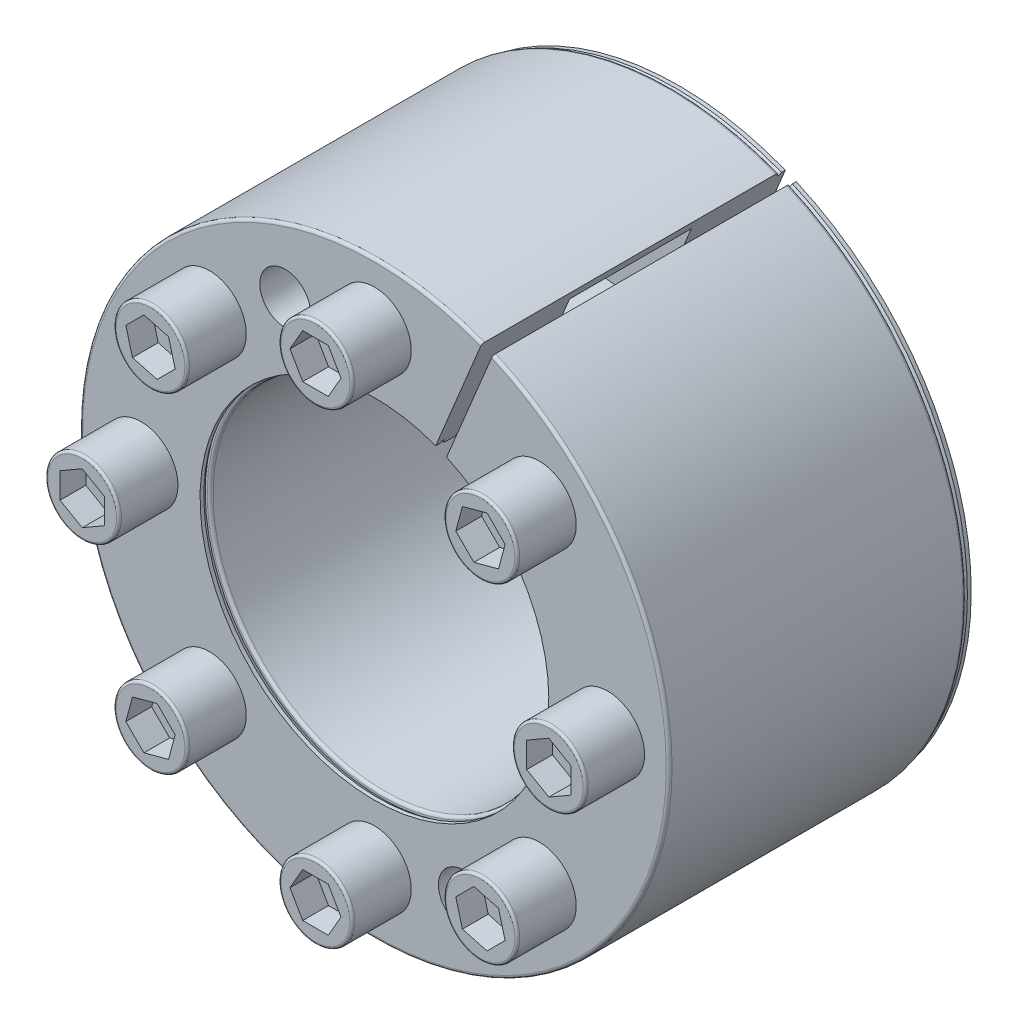
from build123d import *

# Parameters (mm, degrees)
SKETCH7_W                                 = 12.4
SKETCH7_H                                 = 10.625
FILLET2_R                                 = 0.3
SKETCH8_W                                 = 12.4
SKETCH8_H                                 = 3
SCREW_SKETCH1_R                           = 3.75
EXTRUDE_SCREW_SOCKET_HEAD_DEPTH           = 6
FILLET_SCREW_SOCKET_HEAD_R                = 0.25
CUT_SCREW_SOCKET_HEAD_DEPTH               = 2.625
SKETCH5_W                                 = 4.65
SKETCH5_H                                 = 3
CIRPATTERN1_COUNT                         = 8
FILLET_SCREW_SOCKET_HEAD_OF_CIRPATTERN1_R = 0.25
SKETCH6_R                                 = 2.57578125
CUT_EXTRUDE1_DEPTH                        = 9.3
CIRPATTERN2_COUNT                         = 2
CUT_EXTRUDE_THIN1_DEPTH                   = 53.545218679


with BuildPart() as part:
    # Sketch2 → Revolve1 (revolve)
    with BuildSketch(Plane(origin=(0, 0, 0), x_dir=(0, 0, -1), z_dir=(1, 0, 0)), mode=Mode.PRIVATE) as revolve1_sk:
        Polygon((0.775, 17.5), (31, 17.5), (31, 29.75), (30.6125, 29.75), (30.225, 29.5), (30.225, 30), (0, 30), (0, 18), (0, 17.75), (0.3875, 17.75), (0.775, 18), align=None)
    revolve(revolve1_sk.sketch.rotate(Axis((0, 0, 0), (0, 0, -1)), 90), axis=Axis((0, 0, 0), (0, 0, -1)))

    # Sketch7 → Cut-Revolve2 (revolve, cut)
    with BuildSketch(Plane(origin=(0, 0, 0), x_dir=(0, 0, -1), z_dir=(1, 0, 0)), mode=Mode.PRIVATE) as cut_revolve2_sk:
        with Locations((15.5, 23.75)):
            Rectangle(SKETCH7_W, SKETCH7_H)
    revolve(cut_revolve2_sk.sketch.rotate(Axis((0, 0, 0), (0, 0, -1)), 90), axis=Axis((0, 0, 0), (0, 0, -1)), mode=Mode.SUBTRACT)

    # Fillet2
    fillet2_edges = [part.edges().sort_by_distance(p)[0] for p in [
        (-30, 0, 0),
        (-30, 0, -30.225),
        (-17.5, 0, -31),
        (-17.5, 0, -0.775),
    ]]
    fillet(fillet2_edges, radius=FILLET2_R)

    # Sketch8 → Revolve2 (revolve)
    with BuildSketch(Plane(origin=(0, 0, 0), x_dir=(0, 0, -1), z_dir=(1, 0, 0)), mode=Mode.PRIVATE) as revolve2_sk:
        with Locations((15.5, 25.25)):
            Rectangle(SKETCH8_W, SKETCH8_H)
    revolve2 = revolve(revolve2_sk.sketch.rotate(Axis((0, 23.75, -21.7), (0, 0, 1)), 90), axis=Axis((0, 23.75, -21.7), (0, 0, 1)))

    # Screw Sketch1 → Extrude-Screw (socket head) (add)
    with BuildSketch(Plane(origin=(-37.043082829, 76.082538144, 0), x_dir=(1, 0, 0), z_dir=(0, 0, 1))):
        with Locations(Location((37.043082829, -52.332538144, 0), (0, 0, 180))):
            Circle(SCREW_SKETCH1_R)
    extrude_screw_socket_head = extrude(amount=EXTRUDE_SCREW_SOCKET_HEAD_DEPTH)

    # Fillet-Screw (socket head)
    fillet_screw_socket_head_edges = [part.edges().sort_by_distance(p)[0] for p in [
        (3.75, 23.75, 6),
    ]]
    fillet(fillet_screw_socket_head_edges, radius=FILLET_SCREW_SOCKET_HEAD_R)

    # Screw Sketch2 → Cut-Screw (socket head) (cut)
    with BuildSketch(Plane(origin=(0, 82.5, 6), x_dir=(1, 0, 0), z_dir=(0, 0, 1))):
        Polygon((2.598076211, -58.75), (1.299038106, -56.5), (-1.299038106, -56.5), (-2.598076211, -58.75), (-1.299038106, -61), (1.299038106, -61), align=None)
    cut_screw_socket_head = extrude(amount=-CUT_SCREW_SOCKET_HEAD_DEPTH, mode=Mode.SUBTRACT)

    # Sketch5 → Cut-Revolve1 (revolve, cut)
    with BuildSketch(Plane(origin=(0, 0, 0), x_dir=(0, 0, -1), z_dir=(1, 0, 0)), mode=Mode.PRIVATE) as cut_revolve1_sk:
        with Locations((28.675, 25.25)):
            Rectangle(SKETCH5_W, SKETCH5_H)
    cut_revolve1 = revolve(cut_revolve1_sk.sketch.rotate(Axis((0, 23.75, -31), (0, 0, 1)), 270), axis=Axis((0, 23.75, -31), (0, 0, 1)), mode=Mode.SUBTRACT)

    # CirPattern1: Revolve2, Extrude-Screw (socket head), Cut-Screw (socket head), Cut-Revolve1 ×8 about axis
    cirpattern1_axis = Axis((0, 0, 0), (0, 0, 1))
    add([revolve2.rotate(cirpattern1_axis, i * 360 / CIRPATTERN1_COUNT) for i in range(1, CIRPATTERN1_COUNT)])
    add([extrude_screw_socket_head.rotate(cirpattern1_axis, i * 360 / CIRPATTERN1_COUNT) for i in range(1, CIRPATTERN1_COUNT)])
    add([cut_screw_socket_head.rotate(cirpattern1_axis, i * 360 / CIRPATTERN1_COUNT) for i in range(1, CIRPATTERN1_COUNT)], mode=Mode.SUBTRACT)
    add([cut_revolve1.rotate(cirpattern1_axis, i * 360 / CIRPATTERN1_COUNT) for i in range(1, CIRPATTERN1_COUNT)], mode=Mode.SUBTRACT)

    # Fillet-Screw (socket head) of CirPattern1
    fillet_screw_socket_head_of_cirpattern1_edges = [part.edges().sort_by_distance(p)[0] for p in [
        (-14.142135624, 19.445436483, 6),
        (-23.75, 3.75, 6),
        (-19.445436483, -14.142135624, 6),
        (-3.75, -23.75, 6),
        (14.142135624, -19.445436483, 6),
        (23.75, -3.75, 6),
        (19.445436483, 14.142135624, 6),
    ]]
    fillet(fillet_screw_socket_head_of_cirpattern1_edges, radius=FILLET_SCREW_SOCKET_HEAD_OF_CIRPATTERN1_R)

    # Sketch6 → Cut-Extrude1 (cut)
    with BuildSketch(Plane.XY):
        with Locations((-9.088731519, 21.942138897)):
            Circle(SKETCH6_R)
    cut_extrude1 = extrude(amount=-CUT_EXTRUDE1_DEPTH, mode=Mode.SUBTRACT)

    # CirPattern2: Cut-Extrude1 ×2 about axis
    cirpattern2_axis = Axis((0, 0, 0), (0, 0, 1))
    for i in range(1, CIRPATTERN2_COUNT):
        add(cut_extrude1.rotate(cirpattern2_axis, i * 360 / CIRPATTERN2_COUNT), mode=Mode.SUBTRACT)

    # Sketch9 → Cut-Extrude-Thin1 (cut, through all)
    with BuildSketch(Plane.XY):
        Polygon((0.55432772, -0.229610059), (12.03483069, 27.486775916), (10.926175251, 27.945996035), (-0.55432772, 0.229610059), align=None)
    extrude(amount=-CUT_EXTRUDE_THIN1_DEPTH, mode=Mode.SUBTRACT)


solid = part.part
